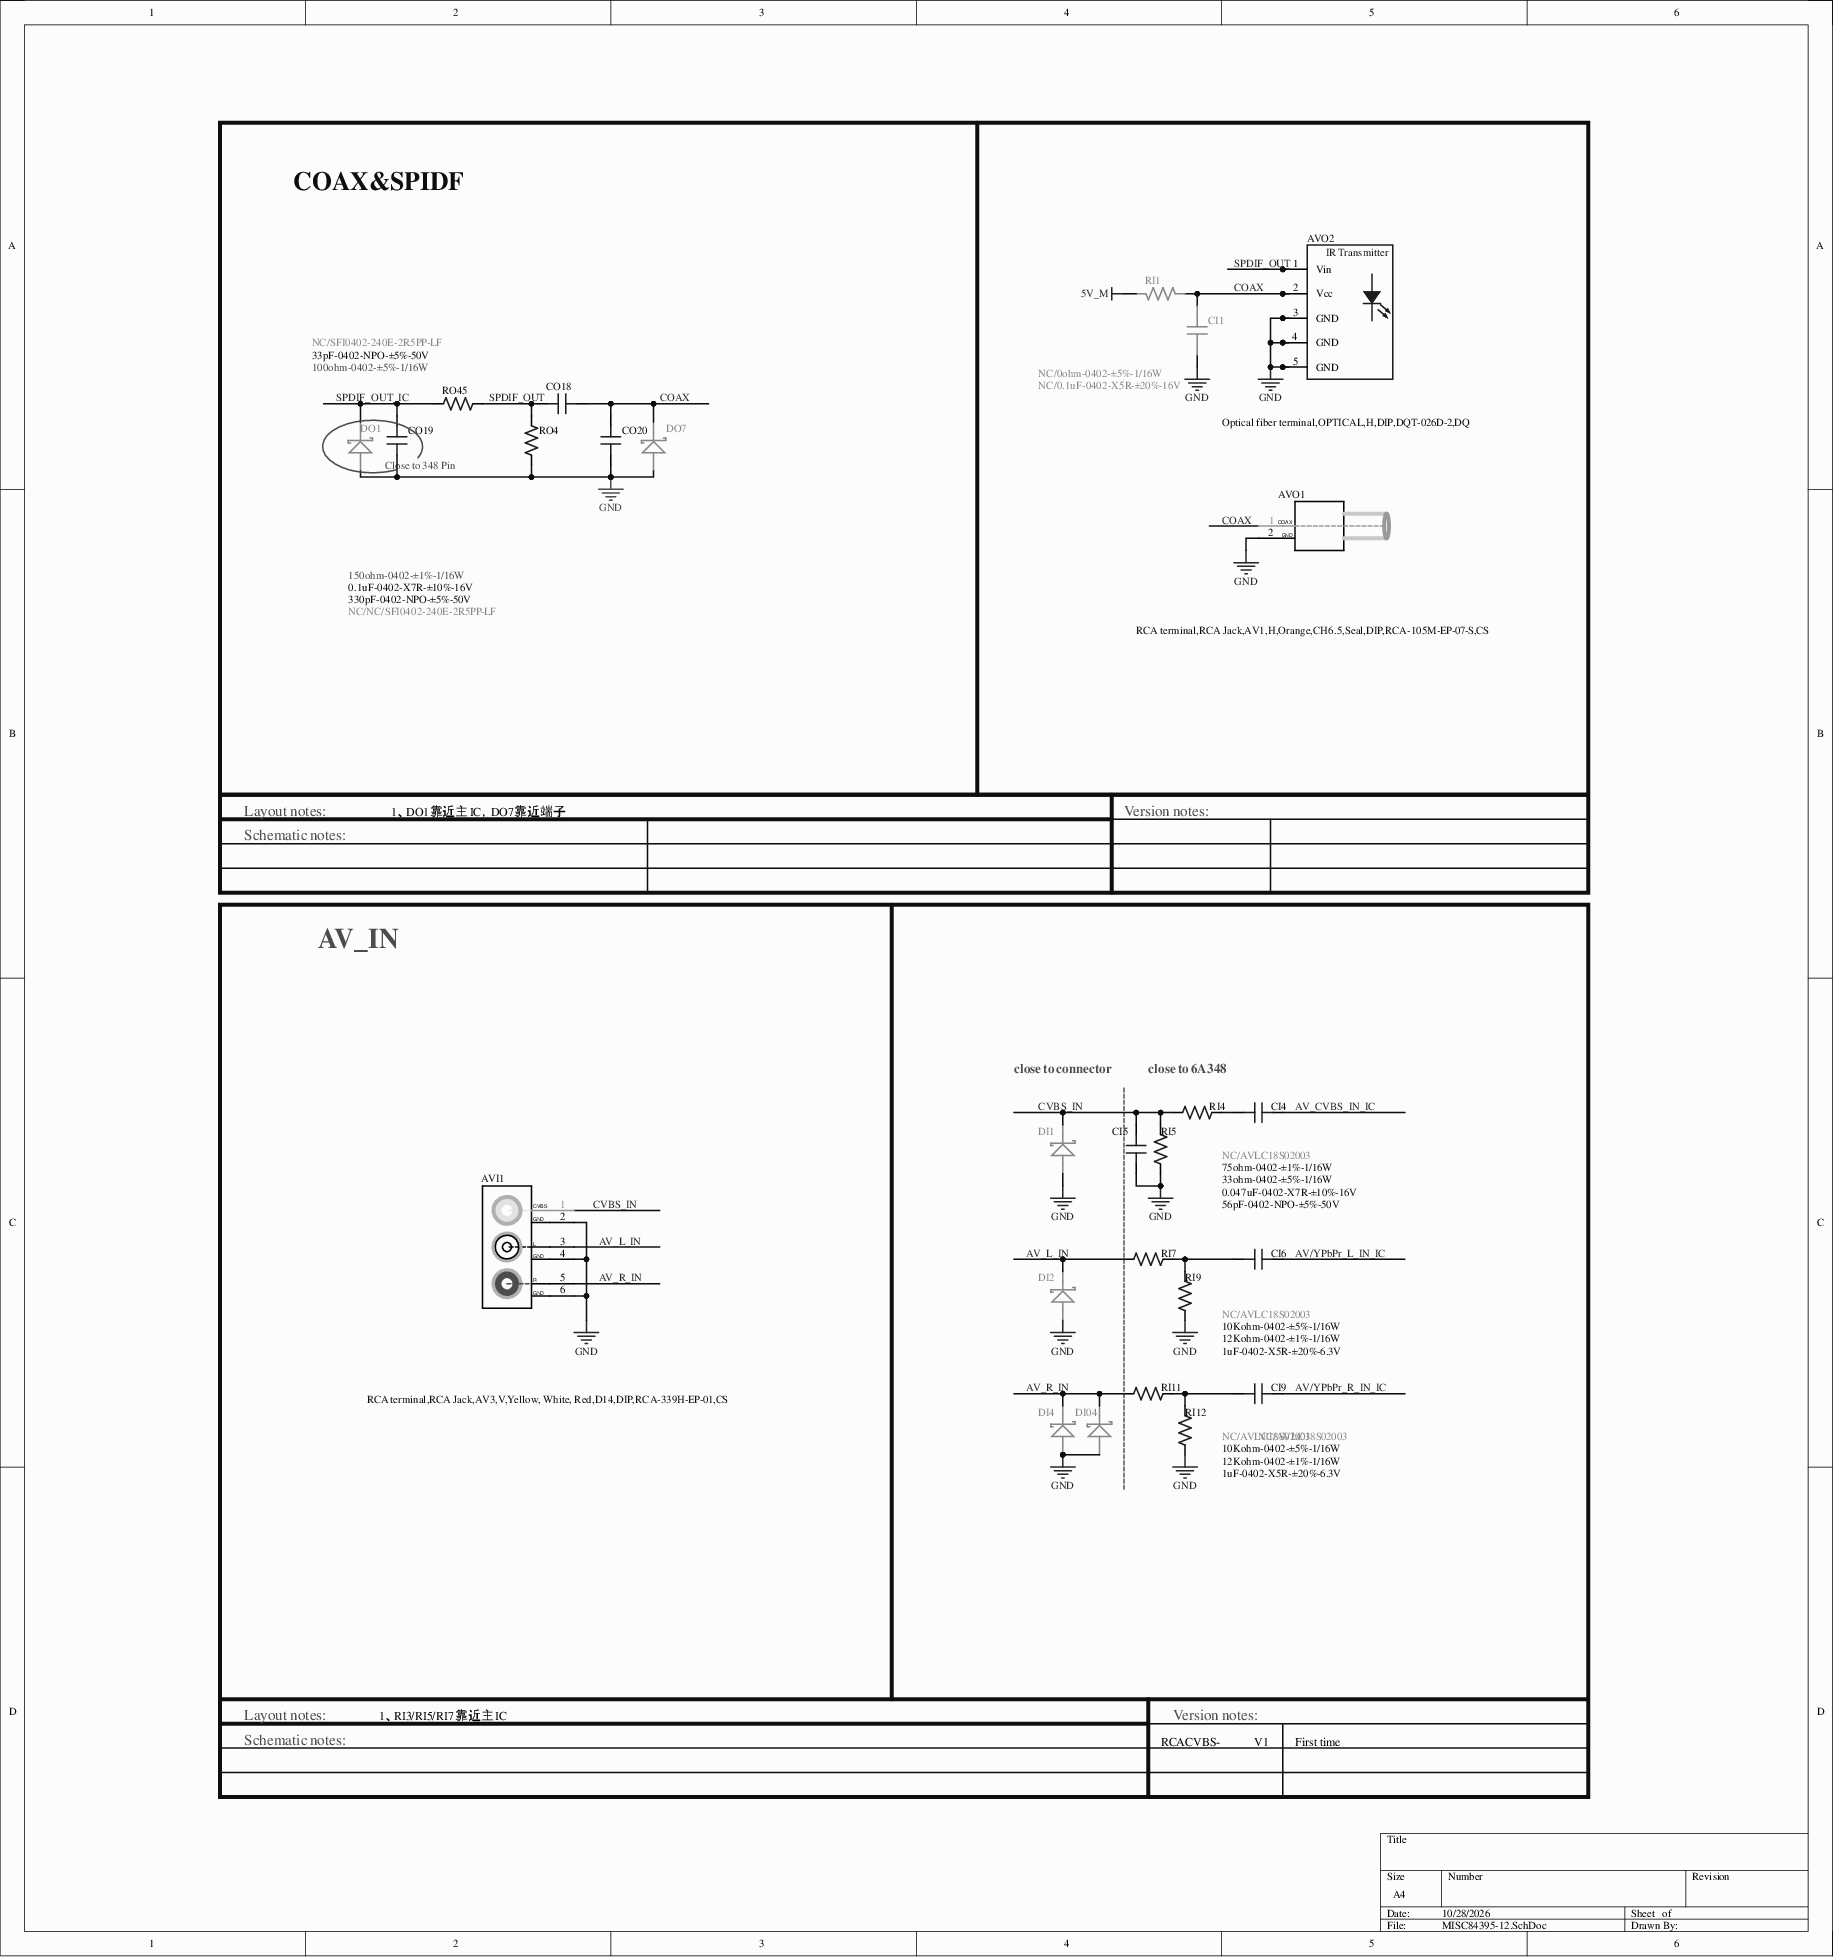
[diagram p0: MISC84395-12.SchDoc]
# Altium project MISC84395-37.PrjPCB (part 8 of 13)

## Sheet MISC84395-12.SchDoc
size 381 x 406 mm

### Parts
AVI1  RCA terminal,RCA Jack,AV3,V,Yellow, White, Red,D14,DIP,RCA-339H-EP-01,CS  [AV3-V14-1]
AVO1  RCA terminal,RCA Jack,AV1,H,Orange,CH6.5,Seal,DIP,RCA-105M-EP-07-S,CS  [AV1-H-1]
AVO2  Optical fiber terminal,OPTICAL,H,DIP,DQT-026D-2,DQ  [OPTICAL-HD-3]
CI1  NC/0.1uF-0402-X5R-±20%-16V  [C0402]
CI4  0.047uF-0402-X7R-±10%-16V  [C0402]
CI5  56pF-0402-NPO-±5%-50V  [C0402]
CI6  1uF-0402-X5R-±20%-6.3V  [C0402]
CI9  1uF-0402-X5R-±20%-6.3V  [C0402]
CO18  0.1uF-0402-X7R-±10%-16V  [C0402]
CO19  33pF-0402-NPO-±5%-50V  [C0402]
CO20  330pF-0402-NPO-±5%-50V  [C0402]
DI1  NC/AVLC18S02003  [DIODE-S0402]
DI2  NC/AVLC18S02003  [DIODE-S0402]
DI4  NC/AVLC18S02003  [DIODE-S0402]
DI04  NC/AVLC18S02003  [DIODE-S0402]
DO1  NC/NC/SFI0402-240E-2R5PP-LF  [DIODE-S0402]
DO7  NC/SFI0402-240E-2R5PP-LF  [DIODE-S0402]
RI1  NC/0ohm-0402-±5%-1/16W  [R0402]
RI4  33ohm-0402-±5%-1/16W  [R0402]
RI5  75ohm-0402-±1%-1/16W  [R0402]
RI7  10Kohm-0402-±5%-1/16W  [R0402]
RI9  12Kohm-0402-±1%-1/16W  [R0402]
RI11  10Kohm-0402-±5%-1/16W  [R0402]
RI12  12Kohm-0402-±1%-1/16W  [R0402]
RO4  150ohm-0402-±1%-1/16W  [R0402]
RO45  100ohm-0402-±5%-1/16W  [R0402]

### Blocks framed on the sheet
COAX&SPIDF: AVO1 AVO2 CI1 CO18-CO20 DO1 DO7 RI1 RO4 RO45
AV_IN: AVI1 CI4-CI6 CI9 DI1 DI2 DI04 DI4 RI4 RI5 RI7 RI9 RI11 RI12

### Nets
5V_M: RI1.1
GND: AVI1.2(GND) AVI1.4 AVI1.6 AVO1.2(GND) AVO2.3(GND) AVO2.4(GND) AVO2.5(GND) CI1.1 CI5.1 CO19.1 CO20.1 DI1.A DI2.A DI4.A DI04.A DO1.A DO7.A RI5.1 RI9.2 RI12.2 RO4.1
AV/YPbPr_L_IN_IC: CI6.2
AV/YPbPr_R_IN_IC: CI9.2
AV_CVBS_IN_IC: CI4.1
AV_L_IN: AVI1.3 DI2.K RI7.2
AV_R_IN: AVI1.5 DI4.K DI04.K RI11.2
COAX: AVO1.1(CVBS) AVO2.2(Vcc) CI1.2 CO18.2 CO20.2 DO7.K RI1.2
CVBS_IN: AVI1.1(R) CI5.2 DI1.K RI4.2 RI5.2
SPDIF_OUT: AVO2.1(Vin) CO18.1 RO4.2 RO45.2
SPDIF_OUT_IC: CO19.2 DO1.K RO45.1
NetCI4_2: CI4.2 RI4.1
NetCI6_1: CI6.1 RI7.1 RI9.1
NetCI9_1: CI9.1 RI11.1 RI12.1

### Notes on the sheet
- (near CO19) Close to 348 Pin
- Layout notes:
- 1、DO1靠近主IC，DO7靠近端子
- Version notes:
- Schematic notes:
- close to connector
- close to 6A348
- 1、RI3/RI5/RI7靠近主IC
- RCACVBS-COMPANY_A-V1
- First time

### Library data of the parts
AVI1 = XXX.XXX.0001407-DHMI: RCA terminal,RCA Jack,AV3,V,Yellow, White, Red,D14,DIP,CYB-3.2-3DL11-1-100(R),YK-DHMI
AVO1 = XXX.XXX.0000032-DLMI: RCA terminal,RCA Jack,AV1,H,Orange,CH6.5,Seal,DIP,AV19-01S-0020,QS-DLMI
AVO2 = XXX.XXX.0001777-DLMI: Optical fiber terminal,OPTICAL,H,DIP,182500191,VAST-DLMI
CI1 = 0.1uF-0402-X5R-±20%-16V-D
CI4 = 0.047uF-0402-X7R-±10%-16V-D
CI5 = 56pF-0402-NPO-±5%-50V-D
CI6 CI9 = 1uF-0402-X5R-±20%-16V-D
CO18 = 0.1uF-0402-Y5V-+80%-20%-16V-D
CO19 = 33pF-0402-NPO-±5%-50V-D
CO20 = 330pF-0402-NPO-±5%-50V-D
DI1 DI2 DI4 DI04 DO1 DO7 = AVLC18S02003-D
RI1 RI7 RI11 = 0ohm-0402-±5%-1/16W-D
RI4 = 100ohm-0402-±5%-1/16W-D
RI5 = 75ohm-0402-±5%-1/16W-D
RI9 RI12 = 47Kohm-0402-±5%-1/16W-D
RO4 = 120ohm-0402-±5%-1/16W-D
RO45 = 180ohm-0402-±5%-1/16W-D

## Sheet MISC84395-13.SchDoc
size 431 x 340 mm
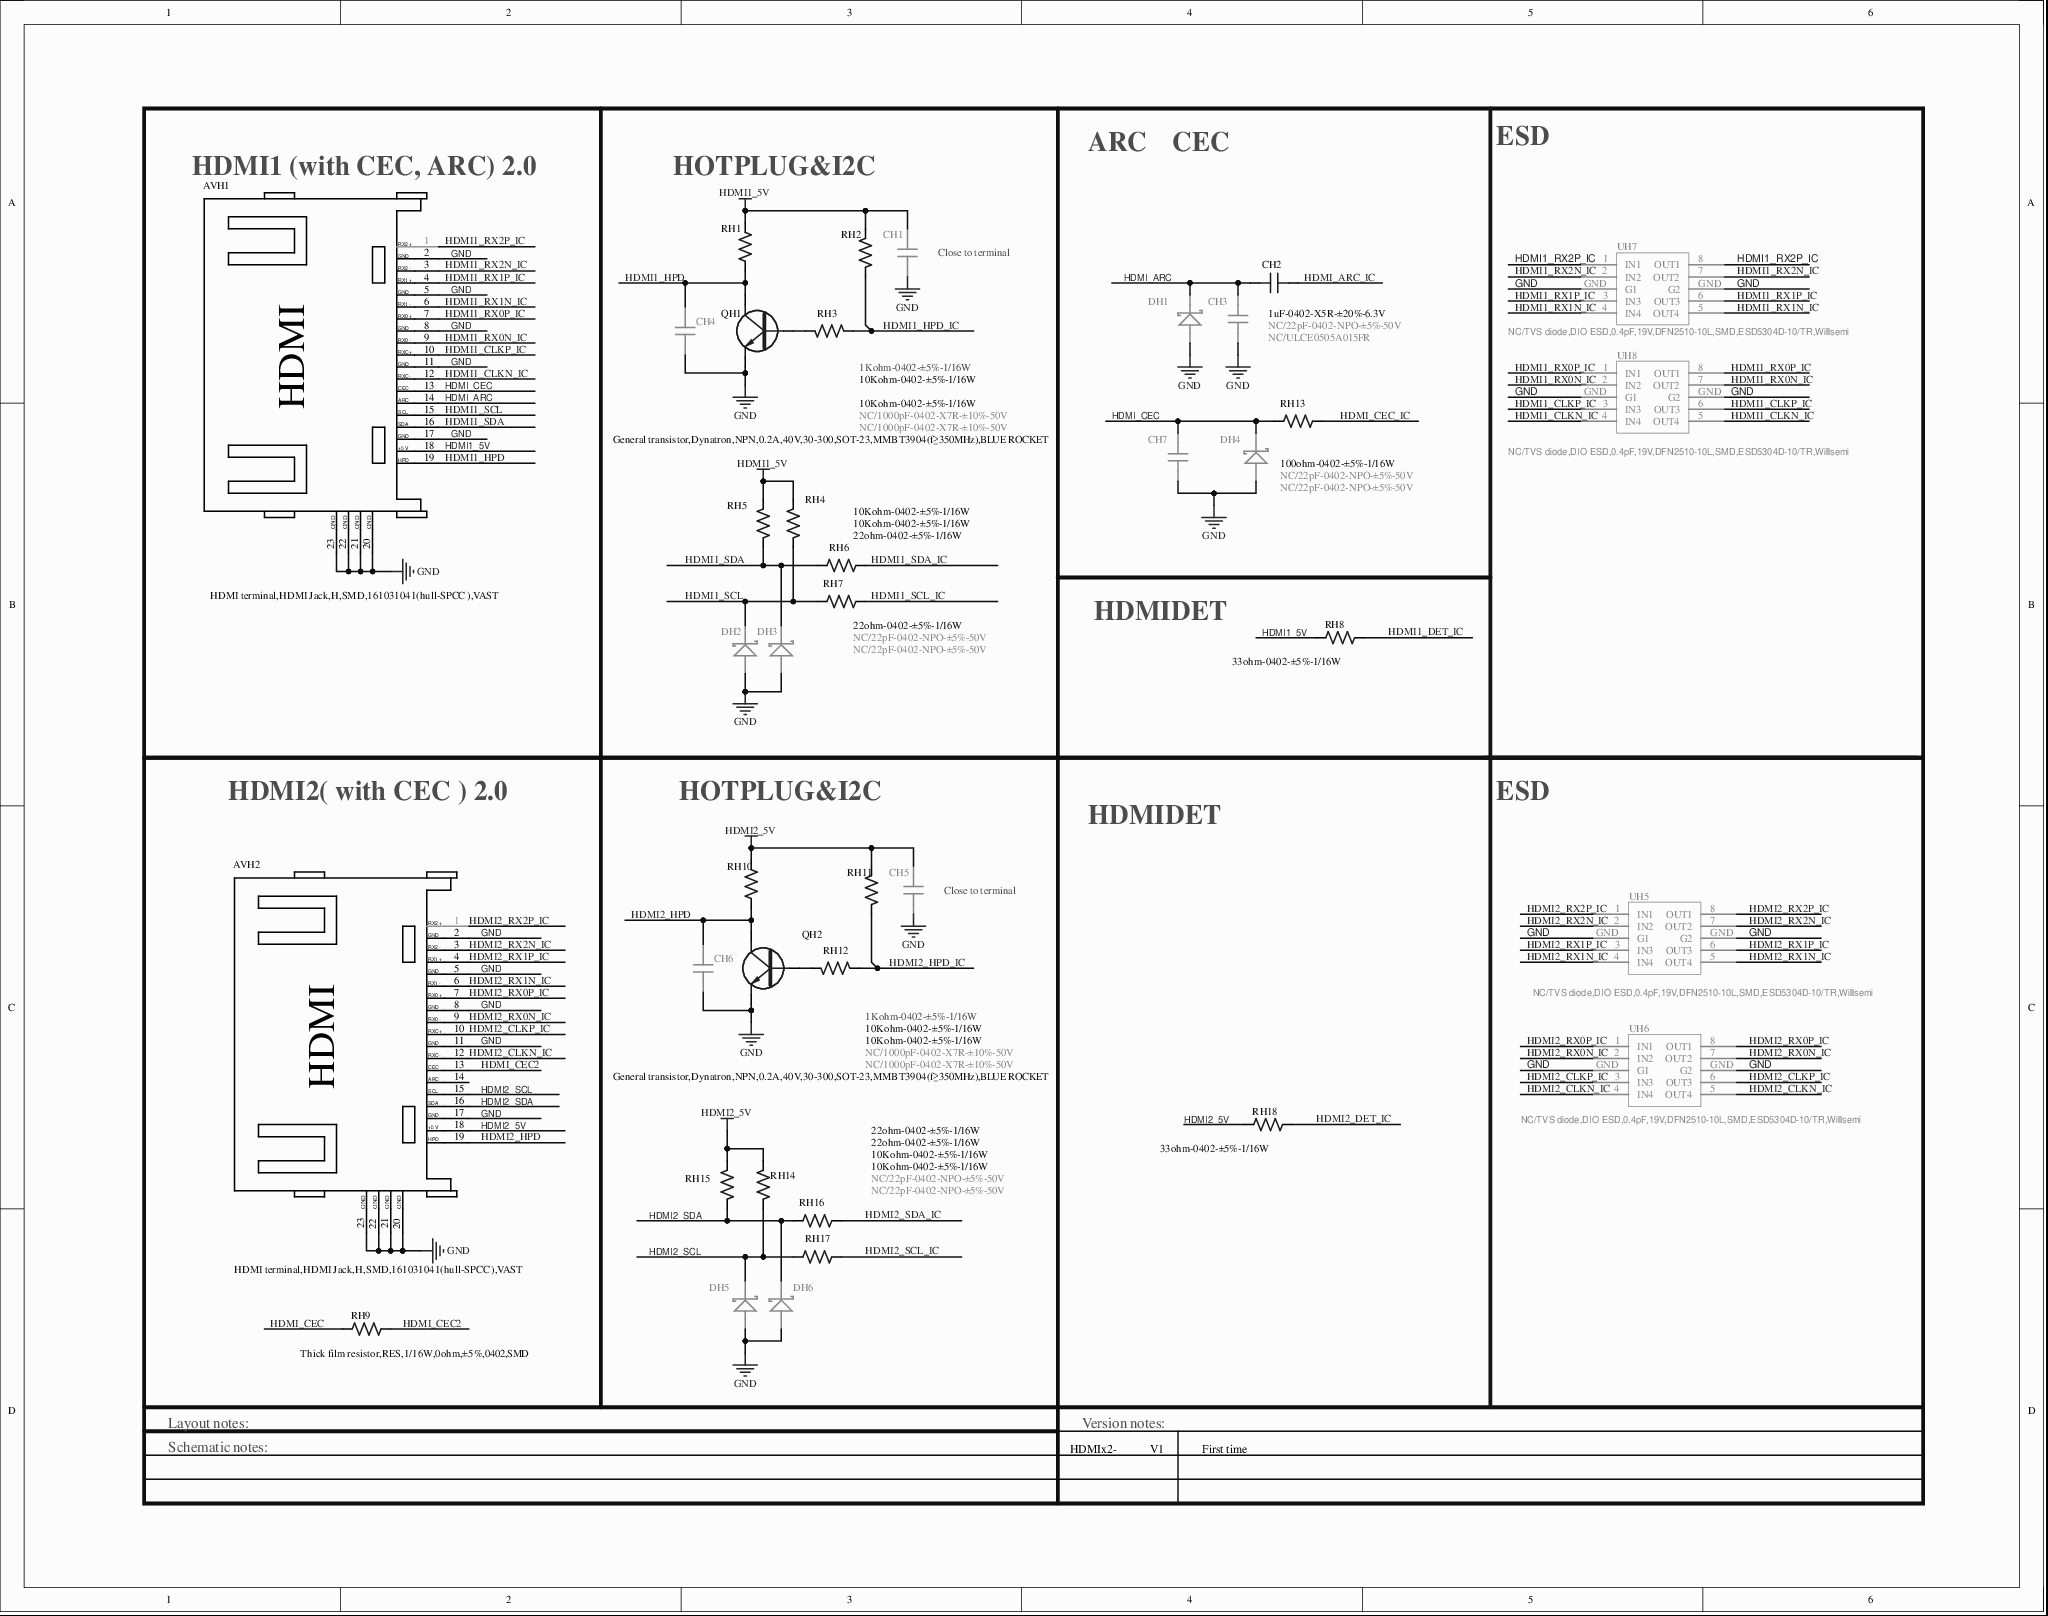
[diagram p1: MISC84395-13.SchDoc]

### Parts
AVH1  HDMI terminal,HDMI Jack,H,SMD,161031041(hull-SPCC ),VAST  [HDMI-HS-1]
AVH2  HDMI terminal,HDMI Jack,H,SMD,161031041(hull-SPCC ),VAST  [HDMI-HS-1]
CH1  NC/1000pF-0402-X7R-±10%-50V  [C0402]
CH2  1uF-0402-X5R-±20%-6.3V  [C0402]
CH3  NC/22pF-0402-NPO-±5%-50V  [C0402]
CH4  NC/1000pF-0402-X7R-±10%-50V  [C0402]
CH5  NC/1000pF-0402-X7R-±10%-50V  [C0402]
CH6  NC/1000pF-0402-X7R-±10%-50V  [C0402]
CH7  NC/22pF-0402-NPO-±5%-50V  [C0402]
DH1  NC/ULCE0505A015FR  [DIODE-S0402]
DH2  NC/22pF-0402-NPO-±5%-50V  [DIODE-S0402]
DH3  NC/22pF-0402-NPO-±5%-50V  [DIODE-S0402]
DH4  NC/22pF-0402-NPO-±5%-50V  [DIODE-S0402]
DH5  NC/22pF-0402-NPO-±5%-50V  [DIODE-S0402]
DH6  NC/22pF-0402-NPO-±5%-50V  [DIODE-S0402]
QH1  General transistor,Dynatron,NPN,0.2A,40V,30-300,SOT-23,MMBT3904(f≥350MHz),BLUE ROCKET  [SOT-23]
QH2  General transistor,Dynatron,NPN,0.2A,40V,30-300,SOT-23,MMBT3904(f≥350MHz),BLUE ROCKET  [SOT-23]
RH1  1Kohm-0402-±5%-1/16W  [R0402]
RH2  10Kohm-0402-±5%-1/16W  [R0402]
RH3  10Kohm-0402-±5%-1/16W  [R0402]
RH4  10Kohm-0402-±5%-1/16W  [R0402]
RH5  10Kohm-0402-±5%-1/16W  [R0402]
RH6  22ohm-0402-±5%-1/16W  [R0402]
RH7  22ohm-0402-±5%-1/16W  [R0402]
RH8  33ohm-0402-±5%-1/16W  [R0402]
RH9  Thick film resistor,RES,1/16W,0ohm,±5%,0402,SMD  [R0402]
RH10  1Kohm-0402-±5%-1/16W  [R0402]
RH11  10Kohm-0402-±5%-1/16W  [R0402]
RH12  10Kohm-0402-±5%-1/16W  [R0402]
RH13  100ohm-0402-±5%-1/16W  [R0402]
RH14  10Kohm-0402-±5%-1/16W  [R0402]
RH15  10Kohm-0402-±5%-1/16W  [R0402]
RH16  22ohm-0402-±5%-1/16W  [R0402]
RH17  22ohm-0402-±5%-1/16W  [R0402]
RH18  33ohm-0402-±5%-1/16W  [R0402]
UH5  NC/TVS diode,DIO ESD,0.4pF,19V,DFN2510-10L,SMD,ESD5304D-10/TR,Willsemi  [RCL0524P]
UH6  NC/TVS diode,DIO ESD,0.4pF,19V,DFN2510-10L,SMD,ESD5304D-10/TR,Willsemi  [RCL0524P]
UH7  NC/TVS diode,DIO ESD,0.4pF,19V,DFN2510-10L,SMD,ESD5304D-10/TR,Willsemi  [RCL0524P]
UH8  NC/TVS diode,DIO ESD,0.4pF,19V,DFN2510-10L,SMD,ESD5304D-10/TR,Willsemi  [RCL0524P]

### Nets
GND: AVH1.2 AVH1.5 AVH1.8 AVH1.11 AVH1.17 AVH1.20 AVH1.21 AVH1.22 AVH1.23 AVH2.2 AVH2.5 AVH2.8 AVH2.11 AVH2.17 AVH2.20 AVH2.21 AVH2.22 AVH2.23 CH1.2 CH3.1 CH4.1 CH5.2 CH6.1 CH7.1 DH1.A DH2.A DH3.A DH4.A DH5.A DH6.A QH1.E QH2.E UH5.GND(G1) UH6.GND(G1) UH7.GND(G1) UH8.GND(G1)
HDMI1_5V: AVH1.18 CH1.1 RH1.1 RH2.1 RH4.1 RH5.1 RH8.1
HDMI2_5V: AVH2.18 CH5.1 RH10.1 RH11.1 RH14.1 RH15.1 RH18.1
HDMI1_CLKN_IC: AVH1.12 UH8.4(IN4) UH8.5(OUT4)
HDMI1_CLKP_IC: AVH1.10 UH8.3(IN3) UH8.6(OUT3)
HDMI1_DET_IC: RH8.2
HDMI1_HPD: AVH1.19 CH4.2 QH1.C RH1.2
HDMI1_HPD_IC: RH2.2 RH3.2
HDMI1_RX0N_IC: AVH1.9 UH8.2(IN2) UH8.7(OUT2)
HDMI1_RX0P_IC: AVH1.7 UH8.1(IN1) UH8.8(OUT1)
HDMI1_RX1N_IC: AVH1.6 UH7.4(IN4) UH7.5(OUT4)
HDMI1_RX1P_IC: AVH1.4 UH7.3(IN3) UH7.6(OUT3)
HDMI1_RX2N_IC: AVH1.3 UH7.2(IN2) UH7.7(OUT2)
HDMI1_RX2P_IC: AVH1.1 UH7.1(IN1) UH7.8(OUT1)
HDMI1_SCL: AVH1.15 DH2.K RH4.2 RH7.1
HDMI1_SCL_IC: RH7.2
HDMI1_SDA: AVH1.16 DH3.K RH5.2 RH6.1
HDMI1_SDA_IC: RH6.2
HDMI2_CLKN_IC: AVH2.12 UH6.4(IN4) UH6.5(OUT4)
HDMI2_CLKP_IC: AVH2.10 UH6.3(IN3) UH6.6(OUT3)
HDMI2_DET_IC: RH18.2
HDMI2_HPD: AVH2.19 CH6.2 QH2.C RH10.2
HDMI2_HPD_IC: RH11.2 RH12.2
HDMI2_RX0N_IC: AVH2.9 UH6.2(IN2) UH6.7(OUT2)
HDMI2_RX0P_IC: AVH2.7 UH6.1(IN1) UH6.8(OUT1)
HDMI2_RX1N_IC: AVH2.6 UH5.4(IN4) UH5.5(OUT4)
HDMI2_RX1P_IC: AVH2.4 UH5.3(IN3) UH5.6(OUT3)
HDMI2_RX2N_IC: AVH2.3 UH5.2(IN2) UH5.7(OUT2)
HDMI2_RX2P_IC: AVH2.1 UH5.1(IN1) UH5.8(OUT1)
HDMI2_SCL: AVH2.15 DH5.K RH14.2 RH17.1
HDMI2_SCL_IC: RH17.2
HDMI2_SDA: AVH2.16 DH6.K RH15.2 RH16.1
HDMI2_SDA_IC: RH16.2
HDMI_ARC: AVH1.14 CH2.1 CH3.2 DH1.K
HDMI_ARC_IC: CH2.2
HDMI_CEC: AVH1.13 CH7.2 DH4.K RH9.2 RH13.1
HDMI_CEC2: AVH2.13 RH9.1
HDMI_CEC_IC: RH13.2
NetQH1_B: QH1.B RH3.1
NetQH2_B: QH2.B RH12.1

Not connected (* = marked no-connect by the designer): AVH2 14*

### Notes on the sheet
- HDMI1 (with CEC, ARC) 2.0
- HOTPLUG&I2C
- ARC
- CEC
- ESD
- (near CH1) Close to terminal
- HDMIDET
- HDMI2( with CEC ) 2.0
- (near CH5) Close to terminal
- Layout notes:
- Schematic notes:
- HDMIx2-COMPANY_A-V1
- Version notes:
- First time

### Library data of the parts
AVH1 AVH2 = HHF-14B000-2SA-H-D-HDMI: CN-HDMI-horizontal-#-#
CH1 CH4-CH6 = 1000pF-0402-X7R-±10%-50V-D
CH2 = 1uF-0402-X5R-±20%-6.3V-D
CH3 CH7 = 22pF-0402-NPO-±5%-50V-D
DH1-DH6 = AVLC18S02003-D
QH1 QH2 = MMBT3904(f≥350MHz)-D-NPN: Q-NPN-#-#-#
RH1 RH10 = 1Kohm-0402-±5%-1/16W-D
RH2-RH5 RH11 RH12 RH14 RH15 = 100ohm-0402-±5%-1/16W-D
RH6 RH7 RH9 RH16 RH17 = 22ohm-0402-±5%-1/16W-D
RH8 RH18 = 33ohm-0402-±5%-1/16W-D
RH13 = 200ohm-0402-±5%-1/16W-D
UH5-UH8 = ULC0524P-D: RCLAMP0524J